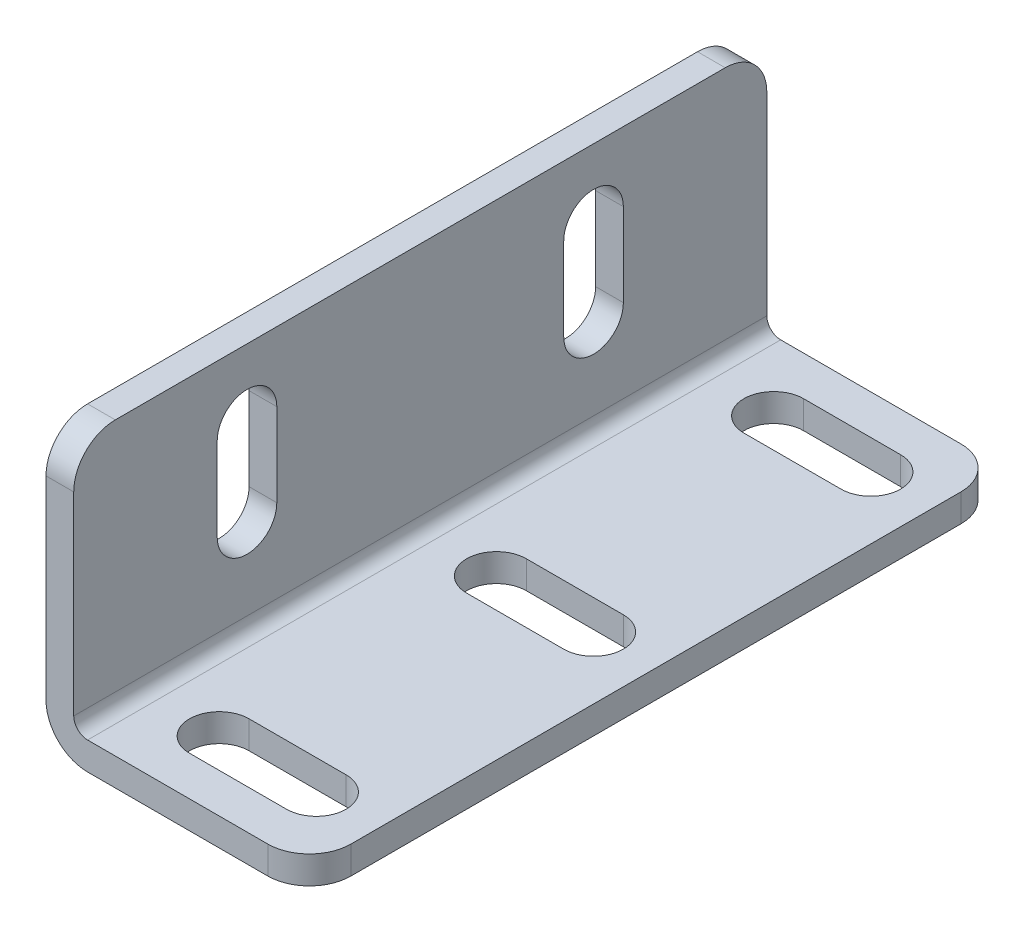
SolidWorks part; units mm, degrees
material "SUS201"
ref_plane "前视基准面" through (0, 0, 0) normal (0, 0, 1) x (1, 0, 0)
ref_plane "上视基准面" through (0, 0, 0) normal (0, 1, 0) x (1, 0, 0)
ref_plane "右视基准面" through (0, 0, 0) normal (1, 0, 0) x (0, 0, -1)
sketch "草图9" plane through (0, 0, 0) normal (0, 0, 1) x (1, 0, 0)
  line L0 (0, 0) -> (0, 18)
  line L1 (0, 0) -> (17, 0)
  dimension "D1" = 17
  dimension "D2" = 18
extrude "拉伸-薄壁1" add sketch "草图9" along normal mid plane 50 thin thin type one direction wall 2
sketch "草图10" plane through (0, 0, 0) normal (0, 1, 0) x (1, 0, 0)
  line L0 (-11.4418, 20) -> (18.3442, 20) construction
  line L1 (5.5, 20) -> (12.5, 20) construction
  line L2 (5.5, 22.15) -> (12.5, 22.15)
  line L3 (5.5, 17.85) -> (12.5, 17.85)
  line L4 (0, 0) -> (41.5624, 0) construction
  line L5 (5.5, -20) -> (12.5, -20) construction
  line L6 (5.5, -22.15) -> (12.5, -22.15)
  line L7 (5.5, -17.85) -> (12.5, -17.85)
  line L8 (17, -25) -> (17, 25) construction
  line L9 (5.5, 0) -> (12.5, 0) construction
  line L10 (5.5, 2.15) -> (12.5, 2.15)
  line L11 (5.5, -2.15) -> (12.5, -2.15)
  arc A0 (5.5, 22.15) -> (5.5, 17.85) centre (5.5, 20) ccw
  arc A1 (12.5, 17.85) -> (12.5, 22.15) centre (12.5, 20) ccw
  arc A2 (5.5, -22.15) -> (5.5, -17.85) centre (5.5, -20) cw
  arc A3 (12.5, -17.85) -> (12.5, -22.15) centre (12.5, -20) cw
  arc A4 (5.5, 2.15) -> (5.5, -2.15) centre (5.5, 0) ccw
  arc A5 (12.5, -2.15) -> (12.5, 2.15) centre (12.5, 0) ccw
  point P4 (9, 20)
  point P14 (9, -20)
  point P23 (9, 0)
  dimension "D4" = 2.15
  dimension "D1" = 7
  dimension "D2" = 8
  dimension "D3" = 20
  dimension "D5" = 2.15
  dimension "D6" = 7
  dimension "D7" = 8
extrude "切除-拉伸1" cut sketch "草图10" against normal blind 10
sketch "草图11" plane through (0, 0, 0) normal (1, 0, 0) x (0, 0, -1)
  line L0 (-12.5, 13) -> (-12.5, 7) construction
  line L1 (-10.35, 13) -> (-10.35, 7)
  line L2 (-14.65, 13) -> (-14.65, 7)
  line L3 (-25, 18) -> (25, 18) construction
  line L4 (0, 0) -> (0, 40.1643) construction
  line L5 (12.5, 13) -> (12.5, 7) construction
  line L6 (10.35, 13) -> (10.35, 7)
  line L7 (14.65, 13) -> (14.65, 7)
  arc A0 (-10.35, 13) -> (-14.65, 13) centre (-12.5, 13) ccw
  arc A1 (-14.65, 7) -> (-10.35, 7) centre (-12.5, 7) ccw
  arc A2 (10.35, 13) -> (14.65, 13) centre (12.5, 13) cw
  arc A3 (14.65, 7) -> (10.35, 7) centre (12.5, 7) cw
  point P2 (-12.5, 10)
  point P14 (12.5, 10)
  dimension "D1" = 2.15
  dimension "D2" = 6
  dimension "D3" = 8
  dimension "D4" = 25
extrude "切除-拉伸2" cut sketch "草图11" against normal blind 10
fillet "圆角1" radius 3 4 edges at (-1, 18, 25) (-1, 18, -25) (17, -1, 25) (17, -1, -25)
fillet "圆角2" radius 1 1 edges at (0, 0, 0)
fillet "圆角3" radius 3 1 edges at (-2, -2, 0)
